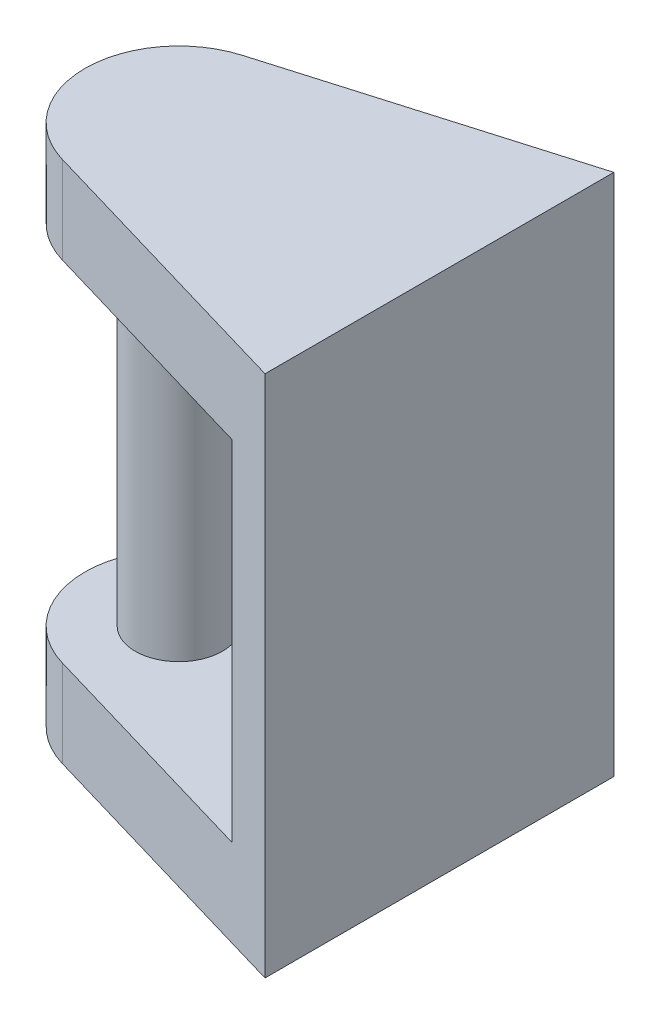
from build123d import *

# Parameters (mm, degrees)
BOSS_EXTRUDE1_DEPTH = 60
CUT_EXTRUDE1_DEPTH  = 40
BOSS_EXTRUDE2_REACH = 77.842
SKETCH3_R           = 5


with BuildPart() as part:
    # Sketch1 → Boss-Extrude1 (new body)
    with BuildSketch(Plane(origin=(0, 0, 0), x_dir=(1, 0, 0), z_dir=(0, 1, 0))):
        with BuildLine():
            Line((0, 0), (0, -40))
            Line((0, -40), (-32.916811342, -30.326541582))
            ThreePointArc((-32.916811342, -30.326541582), (-40.645313725, -20), (-32.916811342, -9.673458418))
            Line((-32.916811342, -9.673458418), (0, 0))
        make_face()
    extrude(amount=BOSS_EXTRUDE1_DEPTH)

    # Sketch2 → Cut-Extrude1 (cut)
    with BuildSketch(Plane(origin=(0, 10, 0), x_dir=(-1, 0, 0), z_dir=(0, -1, 0))):
        with BuildLine():
            Line((5.381519546, -1.581499041), (5.381519546, -38.418500959))
            Line((5.381519546, -38.418500959), (32.916811342, -30.326541582))
            ThreePointArc((32.916811342, -30.326541582), (40.645313725, -20), (32.916811342, -9.673458418))
            Line((32.916811342, -9.673458418), (5.381519546, -1.581499041))
        make_face()
    extrude(amount=-CUT_EXTRUDE1_DEPTH, mode=Mode.SUBTRACT)

    # Sketch3 → Boss-Extrude2 (add, up to next)
    with BuildSketch(Plane(origin=(0, 10, 0), x_dir=(-1, 0, 0), z_dir=(0, -1, 0)), mode=Mode.PRIVATE) as boss_extrude2_sk1:
        with Locations(Location((29.882089371, -20, 0), (0, 0, 90))):
            Circle(SKETCH3_R)
    boss_extrude2_tool1 = extrude(boss_extrude2_sk1.sketch, amount=-BOSS_EXTRUDE2_REACH, mode=Mode.PRIVATE) - part.part
    add(boss_extrude2_tool1.solids().sort_by_distance((-29.882089, 10, 20))[0])


solid = part.part
